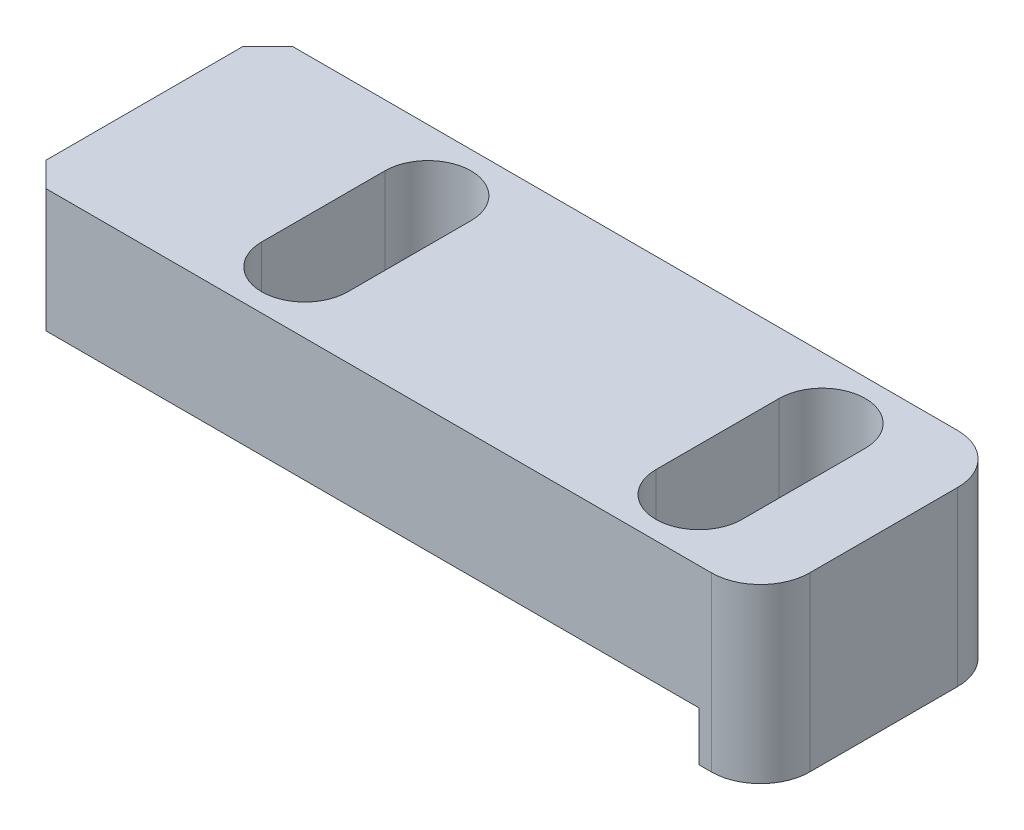
from build123d import *

# Parameters (mm, degrees)
BOSS_EXTRUDE1_DEPTH = 5
CUT_EXTRUDE1_DEPTH  = 31.822070015
FILLET1_R           = 2
CHAMFER1_SIZE       = 1


with BuildPart() as part:
    # Sketch1 → Boss-Extrude1 (new, symmetric)
    with BuildSketch(Plane.XY):
        Polygon((0, 0), (-30, 0), (-30, -5), (-2.5, -5), (-2.5, -7), (0, -7), align=None)
    extrude(amount=BOSS_EXTRUDE1_DEPTH, both=True)

    # Sketch2 → Cut-Extrude1 (cut, through all)
    with BuildSketch(Plane.XZ.offset(5)):
        with BuildLine():
            Line((-19.25, 2.5), (-19.25, -2.5))
            ThreePointArc((-19.25, -2.5), (-21, -4.25), (-22.75, -2.5))
            Line((-22.75, -2.5), (-22.75, 2.5))
            ThreePointArc((-22.75, 2.5), (-21, 4.25), (-19.25, 2.5))
        make_face()
        with BuildLine():
            Line((-3.25, 2.5), (-3.25, -2.5))
            ThreePointArc((-3.25, -2.5), (-5, -4.25), (-6.75, -2.5))
            Line((-6.75, -2.5), (-6.75, 2.5))
            ThreePointArc((-6.75, 2.5), (-5, 4.25), (-3.25, 2.5))
        make_face()
    extrude(amount=-CUT_EXTRUDE1_DEPTH, mode=Mode.SUBTRACT)

    # Fillet1
    fillet1_edges = [part.edges().sort_by_distance(p)[0] for p in [
        (0, -3.5, 5),
        (0, -3.5, -5),
    ]]
    fillet(fillet1_edges, radius=FILLET1_R)

    # Chamfer1
    chamfer1_edges = [part.edges().sort_by_distance(p)[0] for p in [
        (-30, -2.5, 5),
        (-30, -2.5, -5),
    ]]
    chamfer(chamfer1_edges, length=CHAMFER1_SIZE)


solid = part.part
